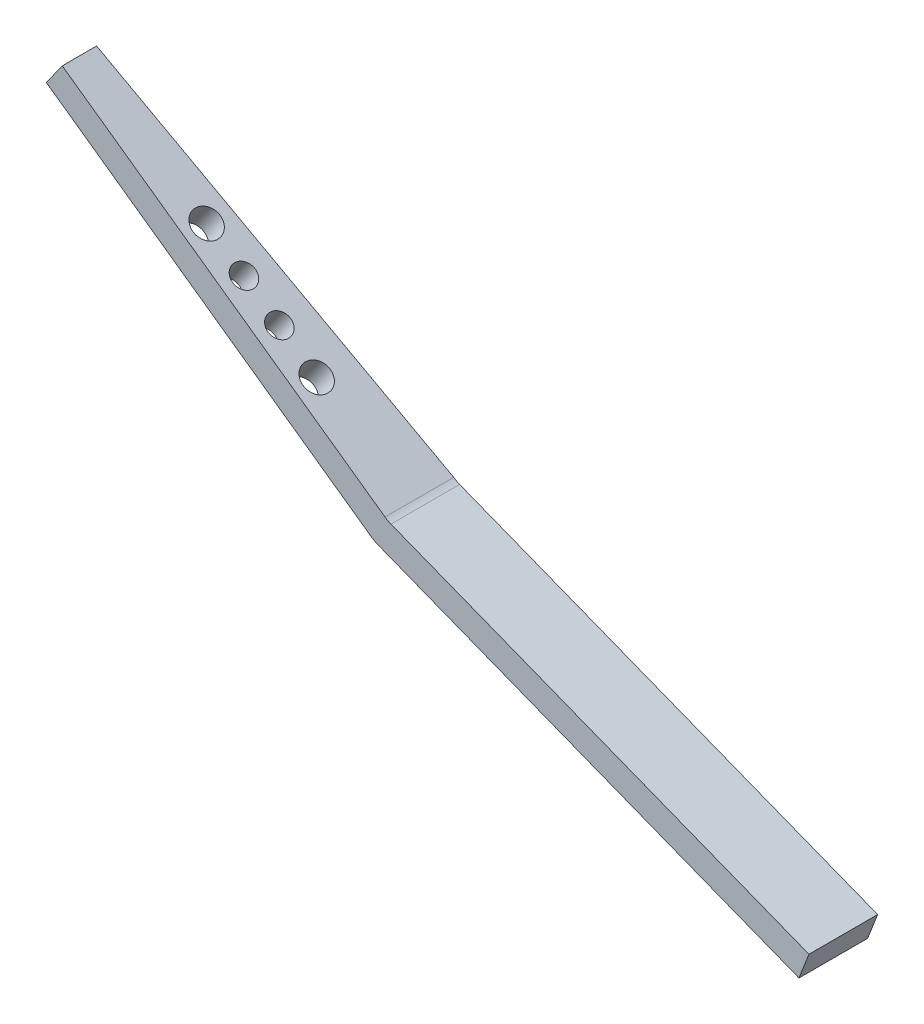
from build123d import *

# Parameters (mm, degrees)
EXTRUDE_1_DEPTH     = 15
CUT_EXTRUDE_1_DEPTH = 237.517683659
SKETCH_5_RX         = 3
SKETCH_5_RY         = 2.999929495
CUT_EXTRUDE_2_DEPTH = 237.517683659
HOLE_WIZARD_M6_1_D  = 5


with BuildPart() as part:
    # 草图1 → 凸台-拉伸1 (new body)
    with BuildSketch(Plane.XY):
        with BuildLine():
            Line((-145.547396155, 197.773537563), (-142.072104357, 202.664585193))
            Line((-142.072104357, 202.664585193), (-71.595844229, 152.588285115))
            ThreePointArc((-71.595844229, 152.588285115), (-70.97220164, 152.200308518), (-70.305827411, 151.891437501))
            Line((-70.305827411, 151.891437501), (20.980591756, 116.19178332))
            Line((20.980591756, 116.19178332), (18.795316776, 110.603888076))
            Line((18.795316776, 110.603888076), (-73.179003731, 146.5725619))
            ThreePointArc((-73.179003731, 146.5725619), (-73.84537796, 146.881432918), (-74.469020549, 147.269409515))
            Line((-74.469020549, 147.269409515), (-145.547396155, 197.773537563))
        make_face()
    extrude(amount=EXTRUDE_1_DEPTH)

    # 草图4 → 切除-拉伸1 (cut, through all)
    with BuildSketch(Plane(origin=(48.026613519, 67.591577297, 0), x_dir=(0.8151746049568697, -0.5792152997231785, 0), z_dir=(0.5792152997231785, 0.8151746049568697, 0))):
        Polygon((-233.2, -7.5), (-146.744583334, 0), (-233.2, 0), align=None)
    extrude(amount=-CUT_EXTRUDE_1_DEPTH, mode=Mode.SUBTRACT)

    # 草图5 → 切除-拉伸2 (cut, through all)
    with BuildSketch(Plane(origin=(48.026613519, 67.591577297, 0), x_dir=(0.8151746049568697, -0.5792152997231785, 0), z_dir=(0.5792152997231785, 0.8151746049568697, 0))):
        with Locations(Location((-171.01991706, -10.129161482), (0, 0, -90))):
            Ellipse(SKETCH_5_RX, SKETCH_5_RY)
        with Locations(Location((-200.50257822, -10.129161482), (0, 0, -90))):
            Ellipse(SKETCH_5_RX, SKETCH_5_RY)
    extrude(amount=-CUT_EXTRUDE_2_DEPTH, mode=Mode.SUBTRACT)

    # M6 螺纹孔1 (through all)
    with Locations(Plane(origin=(48.026613519, 67.591577297, 0), x_dir=(0.8151746049568697, -0.5792152997231785, 0), z_dir=(0.5792152997231785, 0.8151746049568697, 0))):
        with Locations((-181.019682042, -10.129161482), (-190.502813238, -10.129161482)):
            Hole(HOLE_WIZARD_M6_1_D / 2)


solid = part.part
